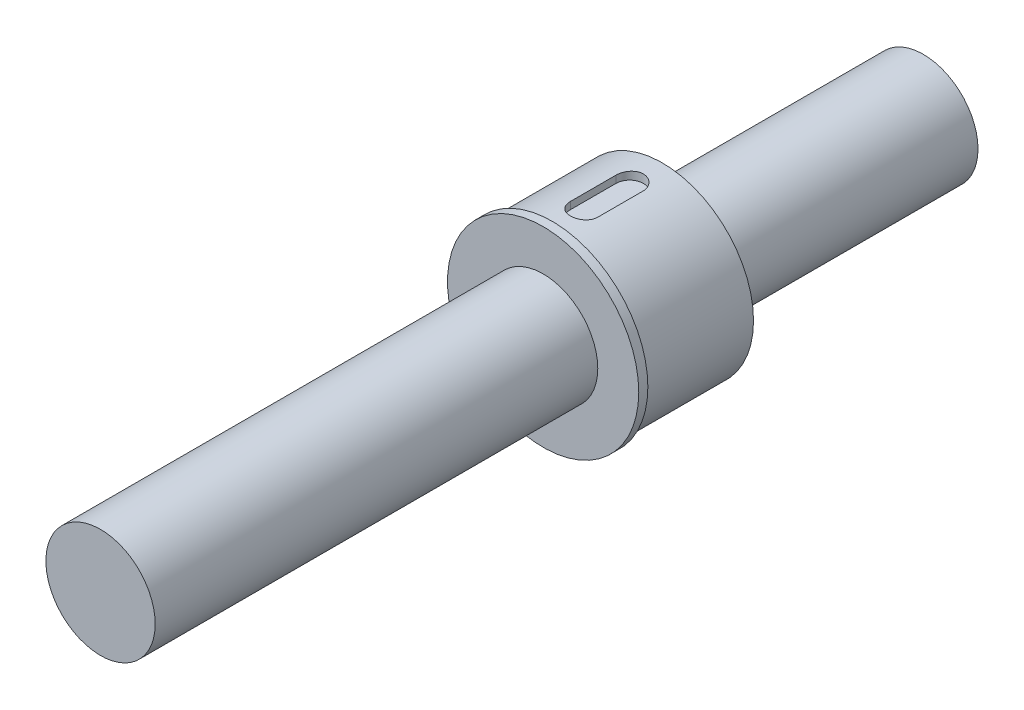
SolidWorks part; units mm, degrees
ref_plane "Front Plane" through (0, 0, 0) normal (0, 0, 1) x (1, 0, 0)
ref_plane "Top Plane" through (0, 0, 0) normal (0, 1, 0) x (1, 0, 0)
ref_plane "Right Plane" through (0, 0, 0) normal (1, 0, 0) x (0, 0, -1)
other "Configuration Table"
sketch "Sketch1" plane through (0, 0, 0) normal (0, 0, 1) x (1, 0, 0)
  circle A0 centre (0, 0) radius 6
  dimension "D1" = 12
extrude "Boss-Extrude1" add sketch "Sketch1" along normal blind 28.65
sketch "Sketch2" plane through (0, 0, 28.65) normal (0, 0, 1) x (1, 0, 0)
  circle A0 centre (0, 0) radius 10
  dimension "D1" = 20
extrude "Boss-Extrude2" add sketch "Sketch2" along normal blind 12.1
sketch "Sketch3" plane through (0, 0, 40.75) normal (0, 0, 1) x (1, 0, 0)
  circle A0 centre (0, 0) radius 10.5
  dimension "D1" = 21
extrude "Boss-Extrude3" add sketch "Sketch3" along normal blind 1
sketch "Sketch4" plane through (0, 0, 41.75) normal (0, 0, 1) x (1, 0, 0)
  circle A0 centre (0, 0) radius 6
  dimension "D1" = 12
extrude "Boss-Extrude4" add sketch "Sketch4" along normal blind 48.6
ref_plane "Plane1" through (0, 6, 0) normal (0, 1, 0) x (1, 0, 0)
ref_plane "Plane2" through (0, 10, 0) normal (0, 1, 0) x (1, 0, 0)
sketch "Sketch6" plane through (0, 10, 0) normal (0, 1, 0) x (1, 0, 0)
  line L0 (0, -10.7624) -> (0, -52.2036) construction
  line L1 (0, -32.25) -> (0, -37.25) construction
  line L2 (1.5, -32.25) -> (1.5, -37.25)
  line L3 (-1.5, -32.25) -> (-1.5, -37.25)
  line L4 (10.5, -40.75) -> (-10.5, -40.75) construction
  line L5 (10.5, -40.75) -> (-10.5, -40.75) construction
  arc A0 (1.5, -32.25) -> (-1.5, -32.25) centre (0, -32.25) ccw
  arc A1 (-1.5, -37.25) -> (1.5, -37.25) centre (0, -37.25) ccw
  point P5 (0, -34.75)
  dimension "D2" = 1.5
  dimension "D1" = 5
  dimension "D3" = 3.5
extrude "Cut-Extrude1" cut sketch "Sketch6" against normal mid plane 1.8
